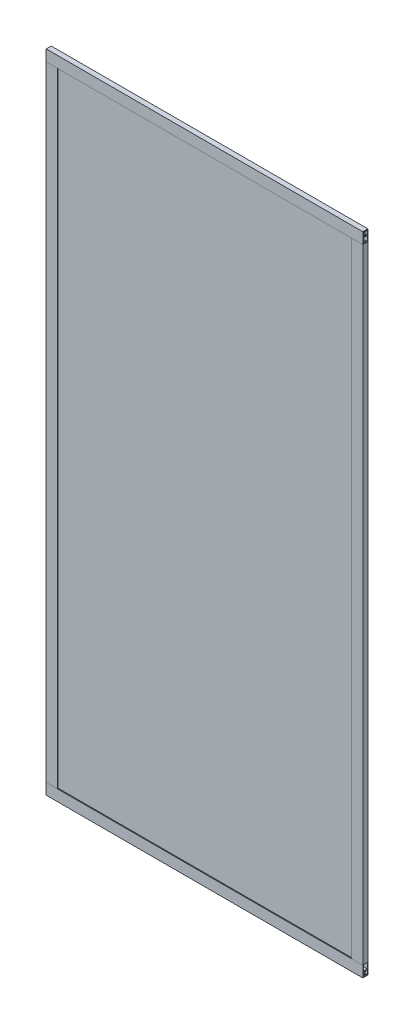
from build123d import *

# Parameters (mm, degrees)
MEMBER_1_DEPTH   = 1135
MEMBER_1_2_DEPTH = 1135
MEMBER_1_3_DEPTH = 2319
MEMBER_1_4_DEPTH = 2319
EXTRUDE_START    = -4
SKETCH_2_W       = 1089
SKETCH_2_H       = 2271
EXTRUDE_1_DEPTH  = 10


with BuildPart() as part:
    # Sketch1 → Member 1 (new body)
    with BuildSketch(Plane(origin=(-567.5, 1158.5, 0), x_dir=(0, 0, -1), z_dir=(1, 0, 0))):
        Polygon((7, -38.5), (5.9, -38.5), (5.9, -40), (7, -40), (9, -40), (9, 0), (-9, 0), (-9, -40), (-7, -40), (-5.9, -40), (-5.9, -38.5), (-7, -38.5), (-7, -20), (7, -20), align=None)
        with BuildLine():
            Line((-1.341640786, -18), (1.341640786, -18))
            ThreePointArc((1.341640786, -18), (1.799302724, -16.749903013), (1.272792206, -15.527207794))
            ThreePointArc((1.272792206, -15.527207794), (1.272792206, -14.749390335), (2.050609665, -14.749390335))
            ThreePointArc((2.050609665, -14.749390335), (2.853462499, -16.282552641), (2.640075756, -18))
            Line((2.640075756, -18), (7, -18))
            Line((7, -18), (7, -3))
            Line((7, -3), (2.640075756, -3))
            ThreePointArc((2.640075756, -3), (2.853462499, -4.717447359), (2.050609665, -6.250609665))
            ThreePointArc((2.050609665, -6.250609665), (1.272792206, -6.250609665), (1.272792206, -5.472792206))
            ThreePointArc((1.272792206, -5.472792206), (1.799302724, -4.250096987), (1.341640786, -3))
            Line((1.341640786, -3), (-1.341640786, -3))
            ThreePointArc((-1.341640786, -3), (-1.799302724, -4.250096987), (-1.272792206, -5.472792206))
            ThreePointArc((-1.272792206, -5.472792206), (-1.272792206, -6.250609665), (-2.050609665, -6.250609665))
            ThreePointArc((-2.050609665, -6.250609665), (-2.853462499, -4.717447359), (-2.640075756, -3))
            Line((-2.640075756, -3), (-7, -3))
            Line((-7, -3), (-7, -18))
            Line((-7, -18), (-2.640075756, -18))
            ThreePointArc((-2.640075756, -18), (-2.853462499, -16.282552641), (-2.050609665, -14.749390335))
            ThreePointArc((-2.050609665, -14.749390335), (-1.272792206, -14.749390335), (-1.272792206, -15.527207794))
            ThreePointArc((-1.272792206, -15.527207794), (-1.799302724, -16.749903013), (-1.341640786, -18))
        make_face(mode=Mode.SUBTRACT)
    extrude(amount=MEMBER_1_DEPTH)


with BuildPart() as body_2:
    # Sketch1 on segment 2 (carried to segment 2) → Member 1 2 (new body)
    with BuildSketch(Plane(origin=(-567.5, -1158.5, 0), x_dir=(0, 0, 1), z_dir=(1, 0, 0))):
        Polygon((7, -38.5), (5.9, -38.5), (5.9, -40), (7, -40), (9, -40), (9, 0), (-9, 0), (-9, -40), (-7, -40), (-5.9, -40), (-5.9, -38.5), (-7, -38.5), (-7, -20), (7, -20), align=None)
        with BuildLine():
            Line((-1.341640786, -18), (1.341640786, -18))
            ThreePointArc((1.341640786, -18), (1.799302724, -16.749903013), (1.272792206, -15.527207794))
            ThreePointArc((1.272792206, -15.527207794), (1.272792206, -14.749390335), (2.050609665, -14.749390335))
            ThreePointArc((2.050609665, -14.749390335), (2.853462499, -16.282552641), (2.640075756, -18))
            Line((2.640075756, -18), (7, -18))
            Line((7, -18), (7, -3))
            Line((7, -3), (2.640075756, -3))
            ThreePointArc((2.640075756, -3), (2.853462499, -4.717447359), (2.050609665, -6.250609665))
            ThreePointArc((2.050609665, -6.250609665), (1.272792206, -6.250609665), (1.272792206, -5.472792206))
            ThreePointArc((1.272792206, -5.472792206), (1.799302724, -4.250096987), (1.341640786, -3))
            Line((1.341640786, -3), (-1.341640786, -3))
            ThreePointArc((-1.341640786, -3), (-1.799302724, -4.250096987), (-1.272792206, -5.472792206))
            ThreePointArc((-1.272792206, -5.472792206), (-1.272792206, -6.250609665), (-2.050609665, -6.250609665))
            ThreePointArc((-2.050609665, -6.250609665), (-2.853462499, -4.717447359), (-2.640075756, -3))
            Line((-2.640075756, -3), (-7, -3))
            Line((-7, -3), (-7, -18))
            Line((-7, -18), (-2.640075756, -18))
            ThreePointArc((-2.640075756, -18), (-2.853462499, -16.282552641), (-2.050609665, -14.749390335))
            ThreePointArc((-2.050609665, -14.749390335), (-1.272792206, -14.749390335), (-1.272792206, -15.527207794))
            ThreePointArc((-1.272792206, -15.527207794), (-1.799302724, -16.749903013), (-1.341640786, -18))
        make_face(mode=Mode.SUBTRACT)
    extrude(amount=MEMBER_1_2_DEPTH)


with BuildPart() as body_3:
    # Sketch1 on segment 3 (carried to segment 3) → Member 1 3 (new body)
    with BuildSketch(Plane(origin=(567.5, 1159.5, 0), x_dir=(0, 0, -1), z_dir=(0, -1, 0))):
        Polygon((7, -38.5), (5.9, -38.5), (5.9, -40), (7, -40), (9, -40), (9, 0), (-9, 0), (-9, -40), (-7, -40), (-5.9, -40), (-5.9, -38.5), (-7, -38.5), (-7, -20), (7, -20), align=None)
        with BuildLine():
            Line((-1.341640786, -18), (1.341640786, -18))
            ThreePointArc((1.341640786, -18), (1.799302724, -16.749903013), (1.272792206, -15.527207794))
            ThreePointArc((1.272792206, -15.527207794), (1.272792206, -14.749390335), (2.050609665, -14.749390335))
            ThreePointArc((2.050609665, -14.749390335), (2.853462499, -16.282552641), (2.640075756, -18))
            Line((2.640075756, -18), (7, -18))
            Line((7, -18), (7, -3))
            Line((7, -3), (2.640075756, -3))
            ThreePointArc((2.640075756, -3), (2.853462499, -4.717447359), (2.050609665, -6.250609665))
            ThreePointArc((2.050609665, -6.250609665), (1.272792206, -6.250609665), (1.272792206, -5.472792206))
            ThreePointArc((1.272792206, -5.472792206), (1.799302724, -4.250096987), (1.341640786, -3))
            Line((1.341640786, -3), (-1.341640786, -3))
            ThreePointArc((-1.341640786, -3), (-1.799302724, -4.250096987), (-1.272792206, -5.472792206))
            ThreePointArc((-1.272792206, -5.472792206), (-1.272792206, -6.250609665), (-2.050609665, -6.250609665))
            ThreePointArc((-2.050609665, -6.250609665), (-2.853462499, -4.717447359), (-2.640075756, -3))
            Line((-2.640075756, -3), (-7, -3))
            Line((-7, -3), (-7, -18))
            Line((-7, -18), (-2.640075756, -18))
            ThreePointArc((-2.640075756, -18), (-2.853462499, -16.282552641), (-2.050609665, -14.749390335))
            ThreePointArc((-2.050609665, -14.749390335), (-1.272792206, -14.749390335), (-1.272792206, -15.527207794))
            ThreePointArc((-1.272792206, -15.527207794), (-1.799302724, -16.749903013), (-1.341640786, -18))
        make_face(mode=Mode.SUBTRACT)
    extrude(amount=MEMBER_1_3_DEPTH)

    # Member 1 3 end butt 1
    split(bisect_by=Plane(origin=(567.5, 1118.5, 0), x_dir=(1, 0, 0), z_dir=(0, -1, 0)), keep=Keep.TOP)

    # Member 1 3 end butt 2
    split(bisect_by=Plane(origin=(567.5, -1118.5, 0), x_dir=(-1, 0, 0), z_dir=(0, 1, 0)), keep=Keep.TOP)


with BuildPart() as body_4:
    # Sketch1 on segment 4 (carried to segment 4) → Member 1 4 (new body)
    with BuildSketch(Plane(origin=(-567.5, 1159.5, 0), x_dir=(0, 0, 1), z_dir=(0, -1, 0))):
        Polygon((7, -38.5), (5.9, -38.5), (5.9, -40), (7, -40), (9, -40), (9, 0), (-9, 0), (-9, -40), (-7, -40), (-5.9, -40), (-5.9, -38.5), (-7, -38.5), (-7, -20), (7, -20), align=None)
        with BuildLine():
            Line((-1.341640786, -18), (1.341640786, -18))
            ThreePointArc((1.341640786, -18), (1.799302724, -16.749903013), (1.272792206, -15.527207794))
            ThreePointArc((1.272792206, -15.527207794), (1.272792206, -14.749390335), (2.050609665, -14.749390335))
            ThreePointArc((2.050609665, -14.749390335), (2.853462499, -16.282552641), (2.640075756, -18))
            Line((2.640075756, -18), (7, -18))
            Line((7, -18), (7, -3))
            Line((7, -3), (2.640075756, -3))
            ThreePointArc((2.640075756, -3), (2.853462499, -4.717447359), (2.050609665, -6.250609665))
            ThreePointArc((2.050609665, -6.250609665), (1.272792206, -6.250609665), (1.272792206, -5.472792206))
            ThreePointArc((1.272792206, -5.472792206), (1.799302724, -4.250096987), (1.341640786, -3))
            Line((1.341640786, -3), (-1.341640786, -3))
            ThreePointArc((-1.341640786, -3), (-1.799302724, -4.250096987), (-1.272792206, -5.472792206))
            ThreePointArc((-1.272792206, -5.472792206), (-1.272792206, -6.250609665), (-2.050609665, -6.250609665))
            ThreePointArc((-2.050609665, -6.250609665), (-2.853462499, -4.717447359), (-2.640075756, -3))
            Line((-2.640075756, -3), (-7, -3))
            Line((-7, -3), (-7, -18))
            Line((-7, -18), (-2.640075756, -18))
            ThreePointArc((-2.640075756, -18), (-2.853462499, -16.282552641), (-2.050609665, -14.749390335))
            ThreePointArc((-2.050609665, -14.749390335), (-1.272792206, -14.749390335), (-1.272792206, -15.527207794))
            ThreePointArc((-1.272792206, -15.527207794), (-1.799302724, -16.749903013), (-1.341640786, -18))
        make_face(mode=Mode.SUBTRACT)
    extrude(amount=MEMBER_1_4_DEPTH)

    # Member 1 4 end butt 1
    split(bisect_by=Plane(origin=(-567.5, 1118.5, 0), x_dir=(1, 0, 0), z_dir=(0, -1, 0)), keep=Keep.TOP)

    # Member 1 4 end butt 2
    split(bisect_by=Plane(origin=(-567.5, -1118.5, 0), x_dir=(-1, 0, 0), z_dir=(0, 1, 0)), keep=Keep.TOP)


with BuildPart() as body_5:
    # 草图2 → 凸台-拉伸1 (new body)
    with BuildSketch(Plane.XY.offset(9).offset(EXTRUDE_START)):
        Rectangle(SKETCH_2_W, SKETCH_2_H)
    extrude(amount=-EXTRUDE_1_DEPTH)


solid = Compound([part.part, body_2.part, body_3.part, body_4.part, body_5.part])
